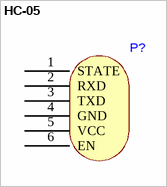
[diagram p0: symbol HC-05]
# Altium schematic symbol library MISC84237-12.SchLib: 1 symbol
Pins are listed as number, name and electrical type; pins without a type are passive.


## HC-05
designator P?
footprint HC-05
pins: 1 STATE, 2 RXD, 3 TXD, 4 GND, 5 VCC, 6 EN